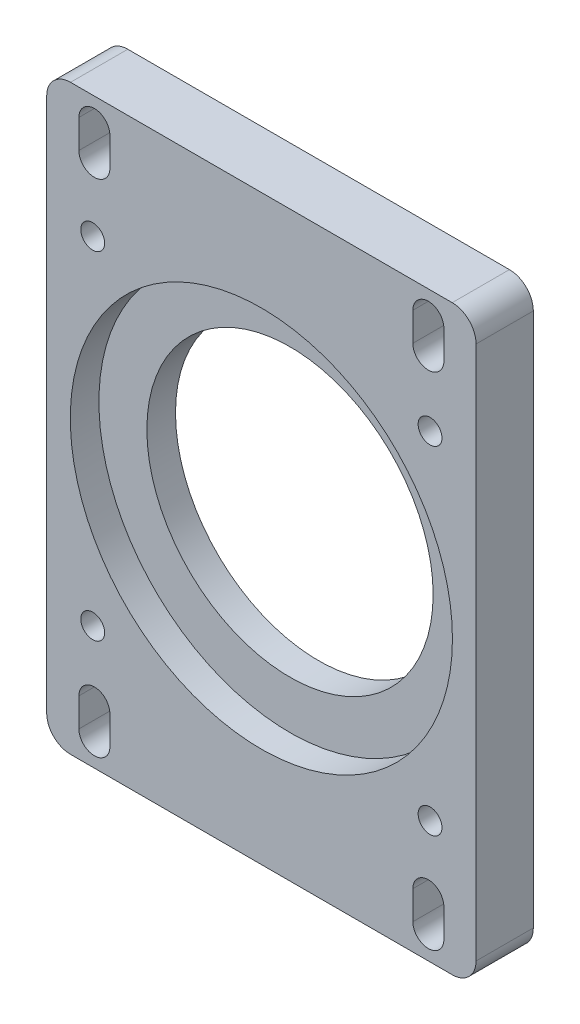
from build123d import *

# Parameters (mm, degrees)
SKETCH1_W           = 90
SKETCH1_H           = 122
BOSS_EXTRUDE1_DEPTH = 12
SKETCH2_R           = 30
CUT_EXTRUDE1_DEPTH  = 77.746335417
SKETCH3_R           = 40.05
CUT_EXTRUDE2_DEPTH  = 6
M6_TAPPED_HOLE1_D   = 5
CUT_EXTRUDE3_DEPTH  = 77.746335417
FILLET1_R           = 5


with BuildPart() as part:
    # Sketch1 → Boss-Extrude1 (new body)
    with BuildSketch(Plane.XY):
        Rectangle(SKETCH1_W, SKETCH1_H)
    extrude(amount=BOSS_EXTRUDE1_DEPTH)

    # Sketch2 → Cut-Extrude1 (cut, through all)
    with BuildSketch(Plane.XY.offset(12)):
        Circle(SKETCH2_R)
    extrude(amount=-CUT_EXTRUDE1_DEPTH, mode=Mode.SUBTRACT)

    # Sketch3 → Cut-Extrude2 (cut)
    with BuildSketch(Plane.XY.offset(12)):
        Circle(SKETCH3_R)
    extrude(amount=-CUT_EXTRUDE2_DEPTH, mode=Mode.SUBTRACT)

    # M6 Tapped Hole1 (through all)
    with Locations(Plane.XY.offset(12)):
        with Locations((35.355339059, 35.355339059), (-35.355339059, 35.355339059), (-35.355339059, -35.355339059), (35.355339059, -35.355339059)):
            Hole(M6_TAPPED_HOLE1_D / 2)

    # Sketch6 → Cut-Extrude3 (cut, through all)
    with BuildSketch(Plane.XY.offset(12)):
        with BuildLine():
            Line((-38.25, 55.5), (-38.25, 49.5))
            ThreePointArc((-38.25, 49.5), (-35, 46.25), (-31.75, 49.5))
            Line((-31.75, 49.5), (-31.75, 55.5))
            ThreePointArc((-31.75, 55.5), (-35, 58.75), (-38.25, 55.5))
        make_face()
        with BuildLine():
            ThreePointArc((38.25, 49.5), (35, 46.25), (31.75, 49.5))
            Line((31.75, 49.5), (31.75, 55.5))
            ThreePointArc((31.75, 55.5), (35, 58.75), (38.25, 55.5))
            Line((38.25, 55.5), (38.25, 49.5))
        make_face()
        with BuildLine():
            Line((38.25, -55.5), (38.25, -49.5))
            ThreePointArc((38.25, -49.5), (35, -46.25), (31.75, -49.5))
            Line((31.75, -49.5), (31.75, -55.5))
            ThreePointArc((31.75, -55.5), (35, -58.75), (38.25, -55.5))
        make_face()
        with BuildLine():
            ThreePointArc((-38.25, -49.5), (-35, -46.25), (-31.75, -49.5))
            Line((-31.75, -49.5), (-31.75, -55.5))
            ThreePointArc((-31.75, -55.5), (-35, -58.75), (-38.25, -55.5))
            Line((-38.25, -55.5), (-38.25, -49.5))
        make_face()
    extrude(amount=-CUT_EXTRUDE3_DEPTH, mode=Mode.SUBTRACT)

    # Fillet1
    fillet1_edges = [part.edges().sort_by_distance(p)[0] for p in [
        (45, -61, 6),
        (-45, -61, 6),
        (-45, 61, 6),
        (45, 61, 6),
    ]]
    fillet(fillet1_edges, radius=FILLET1_R)


solid = part.part
